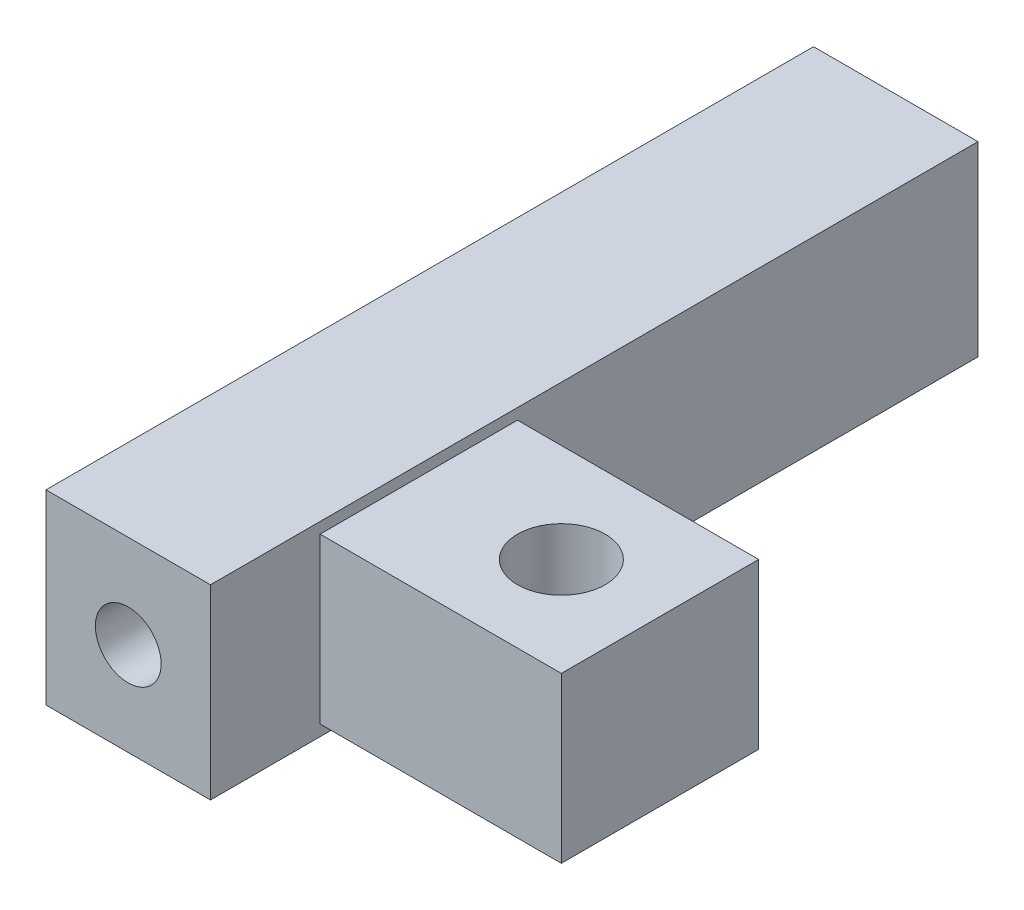
SolidWorks part; units mm, degrees
ref_plane "Front Plane" through (0, 0, 0) normal (0, 0, 1) x (1, 0, 0)
ref_plane "Top Plane" through (0, 0, 0) normal (0, 1, 0) x (1, 0, 0)
ref_plane "Right Plane" through (0, 0, 0) normal (1, 0, 0) x (0, 0, -1)
sketch "Sketch1" plane through (0, 0, 0) normal (0, 0, 1) x (1, 0, 0)
  line L0 (-2, 35) -> (-2, -115) construction
  line L1 (-2, -8.806) -> (-24, -8.806)
  line L2 (-2, -8.806) -> (-2, 6.194)
  line L3 (-2, 6.194) -> (-24, 6.194)
  line L4 (-24, -8.806) -> (-24, 6.194)
  dimension "D1" = 15
  dimension "D2" = 22
extrude "Boss-Extrude1" add sketch "Sketch1" along normal blind 18
sketch "Sketch2" plane through (-24, 0, 0) normal (-1, 0, 0) x (0, 0, 1)
  line L0 (18, -1.306) -> (-7, -1.306) construction
  line L1 (18, 6.194) -> (18, -8.806) construction
  line L3 (-42, 7.194) -> (28, 7.194)
  line L4 (-42, 7.194) -> (-42, -9.806)
  line L5 (-42, -9.806) -> (28, -9.806)
  line L6 (28, 7.194) -> (28, -9.806)
  line L7 (-42, 7.194) -> (28, -9.806) construction
  line L8 (-42, -9.806) -> (28, 7.194) construction
  dimension "D1" = 70
  dimension "D2" = 17
  dimension "D3" = 10
extrude "Boss-Extrude2" add sketch "Sketch2" along normal blind 15
sketch "Sketch3" plane through (0, 6.194, 0) normal (0, 1, 0) x (1, 0, 0)
  circle A0 centre (-11, -9) radius 4
  dimension "D1" = 8
sketch "Sketch4" plane through (0, 0, 28) normal (0, 0, 1) x (1, 0, 0)
  line L0 (-24, -1.306) -> (-39, -1.306) construction
  line L1 (-24, -9.806) -> (-24, 7.194) construction
  line L2 (-39, -9.806) -> (-39, 7.194) construction
  circle A0 centre (-31.5, -1.306) radius 3
  dimension "D1" = 6
extrude "Cut-Extrude2" cut sketch "Sketch4" against normal blind 110
extrude "Cut-Extrude4" cut sketch "Sketch3" against normal blind 41
